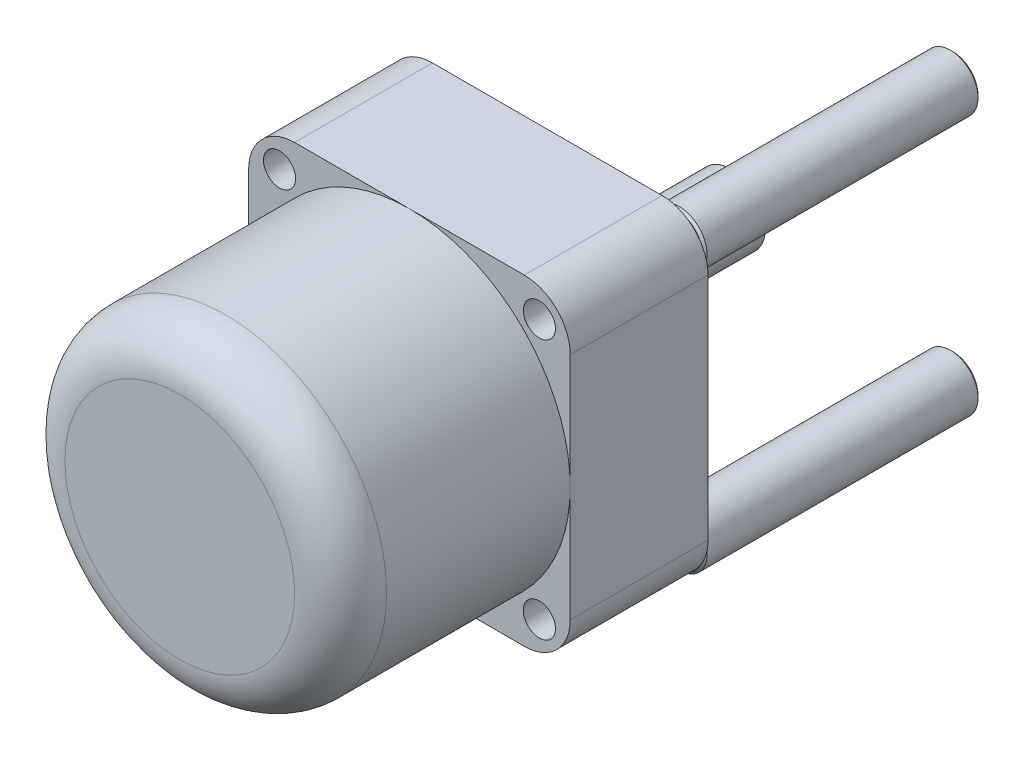
SolidWorks part; units mm, degrees
ref_plane "Front Plane" through (0, 0, 0) normal (0, 0, 1) x (1, 0, 0)
ref_plane "Top Plane" through (0, 0, 0) normal (0, 1, 0) x (1, 0, 0)
ref_plane "Right Plane" through (0, 0, 0) normal (1, 0, 0) x (0, 0, -1)
sketch "Sketch1" plane through (0, 0, 0) normal (0, 0, 1) x (1, 0, 0)
  line L1 (35, -35) -> (-35, -35)
  line L2 (35, -35) -> (35, 35)
  line L3 (35, 35) -> (-35, 35)
  line L4 (-35, -35) -> (-35, 35)
  line L5 (35, -35) -> (-35, 35) construction
  line L6 (35, 35) -> (-35, -35) construction
  point P1 (0, 0)
  dimension "D1" = 70
  dimension "D2" = 70
extrude "Boss-Extrude1" add sketch "Sketch1" along normal blind 30
sketch "Sketch2" plane through (0, 0, 30) normal (0, 0, 1) x (1, 0, 0)
  circle A0 centre (0, 0) radius 27.5
  dimension "D1" = 55
fillet "Fillet2" radius 10 4 edges at (35, -35, 15) (-35, -35, 15) (35, 35, 15) (-35, 35, 15)
sketch "Sketch3" plane through (0, 0, 30) normal (0, 0, 1) x (1, 0, 0)
  line L0 (0, 0) -> (-32.0711, 32.0711) construction
  arc A1 (-25, 35) -> (-35, 25) centre (-25, 25) ccw construction
  circle A2 centre (-28.2843, 28.2843) radius 3.5
  dimension "D2" = 7
extrude "Cut-Extrude1" cut sketch "Sketch3" against normal blind 60
sketch "Sketch4" plane through (0, 0, 0) normal (0, 0, -1) x (-1, 0, 0)
  circle A0 centre (0, 0) radius 22.5
  dimension "D1" = 45
extrude "Boss-Extrude3" add sketch "Sketch4" along normal blind 6
sketch "Sketch5" plane through (0, 0, -6) normal (0, 0, -1) x (-1, 0, 0)
  circle A0 centre (0, 0) radius 7.5
  dimension "D1" = 15
extrude "Boss-Extrude4" add sketch "Sketch5" along normal blind 35
chamfer "Chamfer1" distance 1 angle 45 1 edges at (-7.5, 0, -41)
chamfer "Chamfer2" distance 1 angle 45 1 edges at (-22.5, 0, -6)
pattern_circular "CirPattern1" count 4 over 360 about axis through (0, 0, 0) along (0, 0, 1) of "Cut-Extrude1"
sketch "Sketch6" plane through (0, 0, 30) normal (0, 0, 1) x (1, 0, 0)
  circle A0 centre (0, 0) radius 35
  dimension "D1" = 70
extrude "Boss-Extrude5" add sketch "Sketch6" along normal blind 50
fillet "Fillet3" radius 10 1 edges at (35, 0, 80)
sketch "Sketch7" plane through (0, 0, 0) normal (0, 0, -1) x (-1, 0, 0)
  circle A0 centre (-28.2843, 28.2843) radius 6
  circle A2 centre (28.2843, -28.2843) radius 6
  circle A3 centre (-28.2843, -28.2843) radius 6
  dimension "D1" = 12
extrude "Boss-Extrude6" add sketch "Sketch7" along normal blind 60 separate body
hole_wizard "M6 Tapped Hole1" positions "Sketch8" profile "Sketch9" tap size "M6" standard "GB"
sketch "Sketch8" plane through (0, 0, -60) normal (0, 0, -1) x (-1, 0, 0)
  point P0 (-28.2843, 28.2843)
  point P6 (28.2843, -28.2843)
  point P9 (-28.2843, -28.2843)
sketch "Sketch9" plane through (28.2843, 28.2843, -60) normal (1, 0, 0) x (0, 1, 0)
  line L0 (0, 0) -> (0, 16.5022)
  line L1 (0, 16.5022) -> (2.5, 15)
  line L2 (2.5, 15) -> (2.5, 0)
  line L5 (2.5, 0) -> (0, 0)
  line L10 (0, 16.5022) -> (-2.5, 15) construction
  line L11 (0, -6.35) -> (0, 107.95) construction
  dimension "螺纹孔钻头直径" = 5
  dimension "螺纹孔钻头深度" = 15
  dimension "导头角度" = 118
cosmetic thread "Cosmetic thread 1" parameters "D1"=12, "D2"=6
cosmetic thread "Cosmetic thread 2" parameters "D1"=12, "D2"=6
cosmetic thread "Cosmetic thread 4" parameters "D1"=12, "D2"=6
chamfer "Chamfer3" distance 0.5 angle 45 2 edges at (22.2843, 28.2843, 0) (22.2843, 28.2843, -60)
chamfer "Chamfer5" distance 0.5 angle 45 3 edges at (22.2843, -28.2843, 0) (22.2843, -28.2843, -60) (25.7843, -28.2843, -60)
chamfer "Chamfer6" distance 0.5 angle 45 2 edges at (-34.2843, -28.2843, 0) (-34.2843, -28.2843, -60)
hole_wizard "M6 Tapped Hole2" positions "Sketch12" profile "Sketch11" tap size "M6" standard "GB"
sketch "Sketch12" plane through (0, 0, 0) normal (0, 0, 1) x (1, 0, 0)
  point P0 (28.2843, 28.2843)
  point P3 (-28.2843, -28.2843)
  point P6 (28.2843, -28.2843)
sketch "Sketch11" plane through (28.2843, 28.2843, 0) normal (1, 0, 0) x (0, -1, 0)
  line L0 (0, 0) -> (0, 16.5022)
  line L1 (0, 16.5022) -> (2.5, 15)
  line L2 (2.5, 15) -> (2.5, 0)
  line L5 (2.5, 0) -> (0, 0)
  line L10 (0, 16.5022) -> (-2.5, 15) construction
  line L11 (0, -6.35) -> (0, 107.95) construction
  dimension "螺纹孔钻头直径" = 5
  dimension "螺纹孔钻头深度" = 15
  dimension "导头角度" = 118
cosmetic thread "Cosmetic thread 5" parameters "D1"=12, "D2"=6
cosmetic thread "Cosmetic thread 6" parameters "D1"=12, "D2"=6
cosmetic thread "Cosmetic thread 7" parameters "D1"=12, "D2"=6
